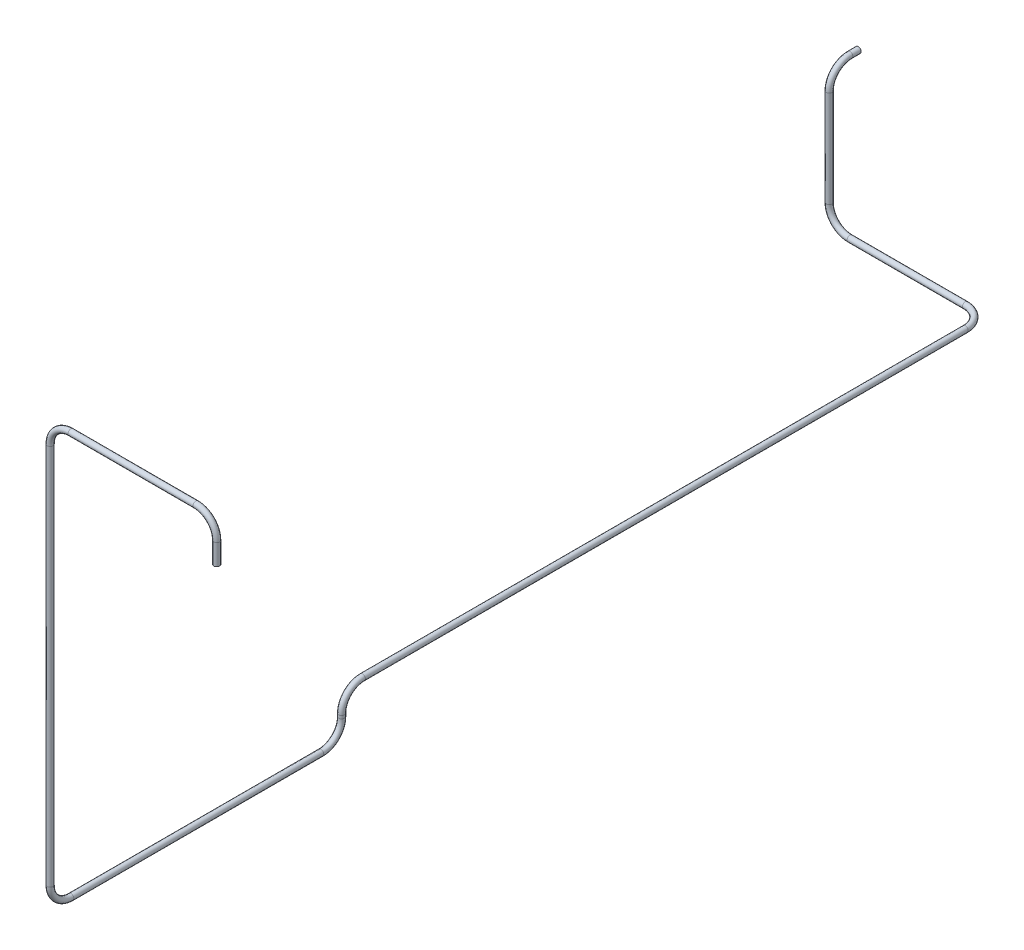
from build123d import *

# Parameters (mm, degrees)
SKETCH_2_R    = 7
SKETCH_2_R_2  = 4
SKETCH_4_R    = 7
SKETCH_4_R_2  = 4
SKETCH_6_R    = 7
SKETCH_6_R_2  = 4
SKETCH_8_R    = 7
SKETCH_8_R_2  = 4
SKETCH_10_R   = 7
SKETCH_10_R_2 = 4


with BuildPart() as part:
    # Sweep 1: sweep along a path in Sketch 1
    with BuildLine(Plane.XY) as sweep_1_path:
        Line((200, 0), (200, 50))
        ThreePointArc((200, 50), (185.355339059, 85.355339059), (150, 100))
        Line((150, 100), (-150, 100))
        ThreePointArc((-150, 100), (-185.355339059, 85.355339059), (-200, 50))
        Line((-200, 50), (-200, -816.5))
    # Sketch 2 → Sweep 1 (sweep)
    with BuildSketch(Plane(origin=(0, 0, 0), x_dir=(1, 0, 0), z_dir=(0, 1, 0))):
        with Locations((200, 0)):
            Circle(SKETCH_2_R)
        with Locations((200, 0)):
            Circle(SKETCH_2_R_2, mode=Mode.SUBTRACT)
    sweep(path=sweep_1_path.line)

    # Sweep 2: sweep along a path in Sketch 3
    with BuildLine(Plane(origin=(-200, 0, 0), x_dir=(0, 0, -1), z_dir=(1, 0, 0))) as sweep_2_path:
        Line((0, -816.5), (0, -866.5))
        ThreePointArc((0, -866.5), (14.644660941, -901.855339059), (50, -916.5))
        Line((50, -916.5), (650, -916.5))
        ThreePointArc((650, -916.5), (685.355339059, -901.855339059), (700, -866.5))
        Line((700, -866.5), (700, -859.5))
        ThreePointArc((700, -859.5), (714.644660941, -824.144660941), (750, -809.5))
        Line((750, -809.5), (2147.5, -809.5))
    # Sketch 4 → Sweep 2 (sweep)
    with BuildSketch(Plane.XZ.offset(816.5)):
        with Locations((-200, 0)):
            Circle(SKETCH_4_R)
        with Locations((-200, 0)):
            Circle(SKETCH_4_R_2, mode=Mode.SUBTRACT)
    sweep(path=sweep_2_path.line)

    # Sweep 3: sweep along a path in Sketch 5
    with BuildLine(Plane(origin=(0, -809.5, 0), x_dir=(1, 0, 0), z_dir=(0, 1, 0))) as sweep_3_path:
        Line((-200, 2147.5), (-200, 2197.5))
        ThreePointArc((-200, 2197.5), (-214.644660941, 2232.855339059), (-250, 2247.5))
        Line((-250, 2247.5), (-449.9, 2247.5))
    # Sketch 6 → Sweep 3 (sweep)
    with BuildSketch(Plane(origin=(0, 0, -2147.5), x_dir=(-1, 0, 0), z_dir=(0, 0, -1))):
        with Locations((200, -809.5)):
            Circle(SKETCH_6_R)
        with Locations((200, -809.5)):
            Circle(SKETCH_6_R_2, mode=Mode.SUBTRACT)
    sweep(path=sweep_3_path.line)

    # Sweep 4: sweep along a path in Sketch 7
    with BuildLine(Plane.XY.offset(-2247.5)) as sweep_4_path:
        Line((-449.9, -809.5), (-526.937126848, -809.5))
        ThreePointArc((-526.937126848, -809.5), (-562.292465907, -794.855339059), (-576.937126848, -759.5))
        Line((-576.937126848, -759.5), (-576.937126848, -577.5))
    # Sketch 8 → Sweep 4 (sweep)
    with BuildSketch(Plane.ZY.offset(449.9)):
        with Locations((-2247.5, -809.5)):
            Circle(SKETCH_8_R)
        with Locations((-2247.5, -809.5)):
            Circle(SKETCH_8_R_2, mode=Mode.SUBTRACT)
    sweep(path=sweep_4_path.line)

    # Sweep 5: sweep along a path in Sketch 9
    with BuildLine(Plane(origin=(-576.937126848, 0, 0), x_dir=(0, 0, -1), z_dir=(1, 0, 0))) as sweep_5_path:
        Line((2247.5, -577.5), (2247.5, -527.5))
        ThreePointArc((2247.5, -527.5), (2262.144660941, -492.144660941), (2297.5, -477.5))
        Line((2297.5, -477.5), (2317.5, -477.5))
    # Sketch 10 → Sweep 5 (sweep)
    with BuildSketch(Plane(origin=(0, -577.5, 0), x_dir=(1, 0, 0), z_dir=(0, 1, 0))):
        with Locations((-576.937126848, 2247.5)):
            Circle(SKETCH_10_R)
        with Locations((-576.937126848, 2247.5)):
            Circle(SKETCH_10_R_2, mode=Mode.SUBTRACT)
    sweep(path=sweep_5_path.line)


solid = part.part
